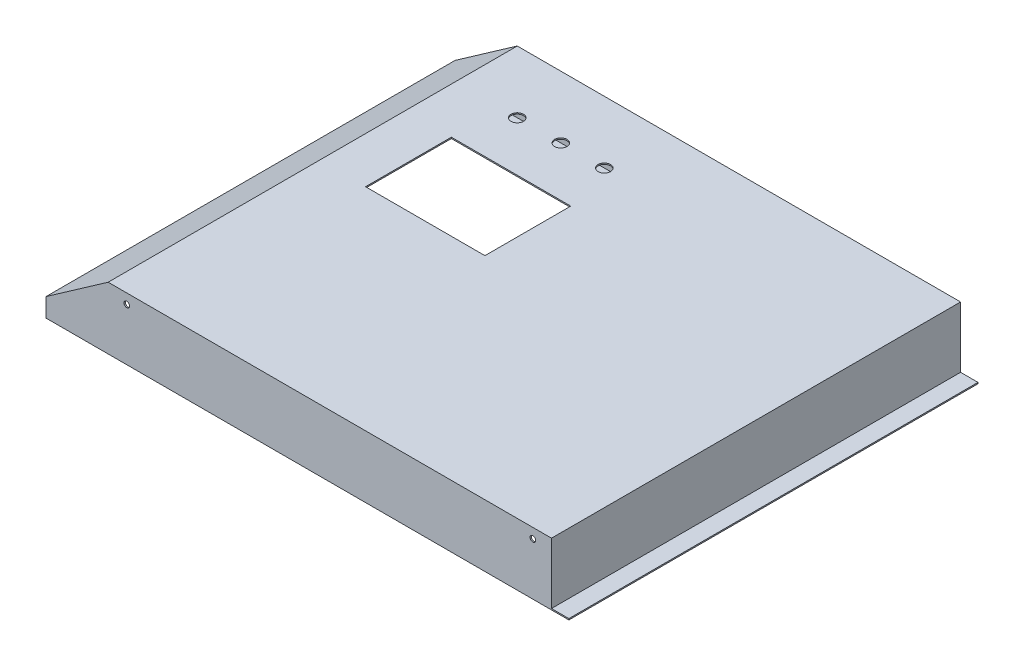
from build123d import *

# Parameters (mm, degrees)
EXTRUDE_1_DEPTH     = 329
SHELL_1_T           = -2
SKETCH_2_R          = 10
SKETCH_2_W          = 192
SKETCH_2_H          = 138
CUT_EXTRUDE_1_DEPTH = 658
SKETCH_3_W          = 30
SKETCH_3_H          = 658
EXTRUDE_2_DEPTH     = 2
EXTRUDE_3_DEPTH     = 2
SKETCH_5_R          = 4.5
CUT_EXTRUDE_2_DEPTH = 797
SKETCH_6_R          = 4.5
CUT_EXTRUDE_3_DEPTH = 10


with BuildPart() as part:
    # 草图1 → 凸台-拉伸1 (new, symmetric)
    with BuildSketch(Plane.XY):
        Polygon((0, 0), (-813, 0), (-813, 30), (-713.029639528, 100), (0, 100), align=None)
    extrude(amount=EXTRUDE_1_DEPTH, both=True)

    # 抽壳1
    shell_1_openings = [part.faces().sort_by_distance(p)[0] for p in [
        (-406.5, 0, 0),
    ]]
    offset(amount=SHELL_1_T, openings=shell_1_openings, kind=Kind.INTERSECTION)

    # 草图2 → 切除-拉伸1 (cut)
    with BuildSketch(Plane(origin=(0, 100, 0), x_dir=(1, 0, 0), z_dir=(0, 1, 0))):
        with Locations(Location((-613.029639528, 229, 0), (0, 0, 180))):
            Circle(SKETCH_2_R)
        with Locations(Location((-543.029639528, 229, 0), (0, 0, 180))):
            Circle(SKETCH_2_R)
        with Locations((-473.029639528, 229)):
            Circle(SKETCH_2_R)
        with Locations((-543.029639528, 80)):
            Rectangle(SKETCH_2_W, SKETCH_2_H)
    extrude(amount=-CUT_EXTRUDE_1_DEPTH, mode=Mode.SUBTRACT)

    # 草图3 → 凸台-拉伸2 (add)
    with BuildSketch(Plane.XZ):
        with Locations((13, 0)):
            Rectangle(SKETCH_3_W, SKETCH_3_H)
    extrude(amount=-EXTRUDE_2_DEPTH)

    # 草图4 → 凸台-拉伸3 (add)
    with BuildSketch(Plane.XZ):
        Polygon((-783, 299), (-783, -299), (0, -299), (0, -329), (-813, -329), (-813, 329), (0, 329), (0, 299), align=None)
    extrude(amount=-EXTRUDE_3_DEPTH)

    # 草图5 → 切除-拉伸2 (cut)
    with BuildSketch(Plane.XY.offset(329)):
        with Locations((-683.029639528, 84)):
            Circle(SKETCH_5_R)
        with Locations((-30, 84)):
            Circle(SKETCH_5_R)
    extrude(amount=-CUT_EXTRUDE_2_DEPTH, mode=Mode.SUBTRACT)

    # 草图6 → 切除-拉伸3 (cut)
    with BuildSketch(Plane.XZ):
        with Locations((-797, 299)):
            Circle(SKETCH_6_R)
        with Locations((-797, -299)):
            Circle(SKETCH_6_R)
        with Locations((-797, 0)):
            Circle(SKETCH_6_R)
    extrude(amount=-CUT_EXTRUDE_3_DEPTH, mode=Mode.SUBTRACT)


solid = part.part
